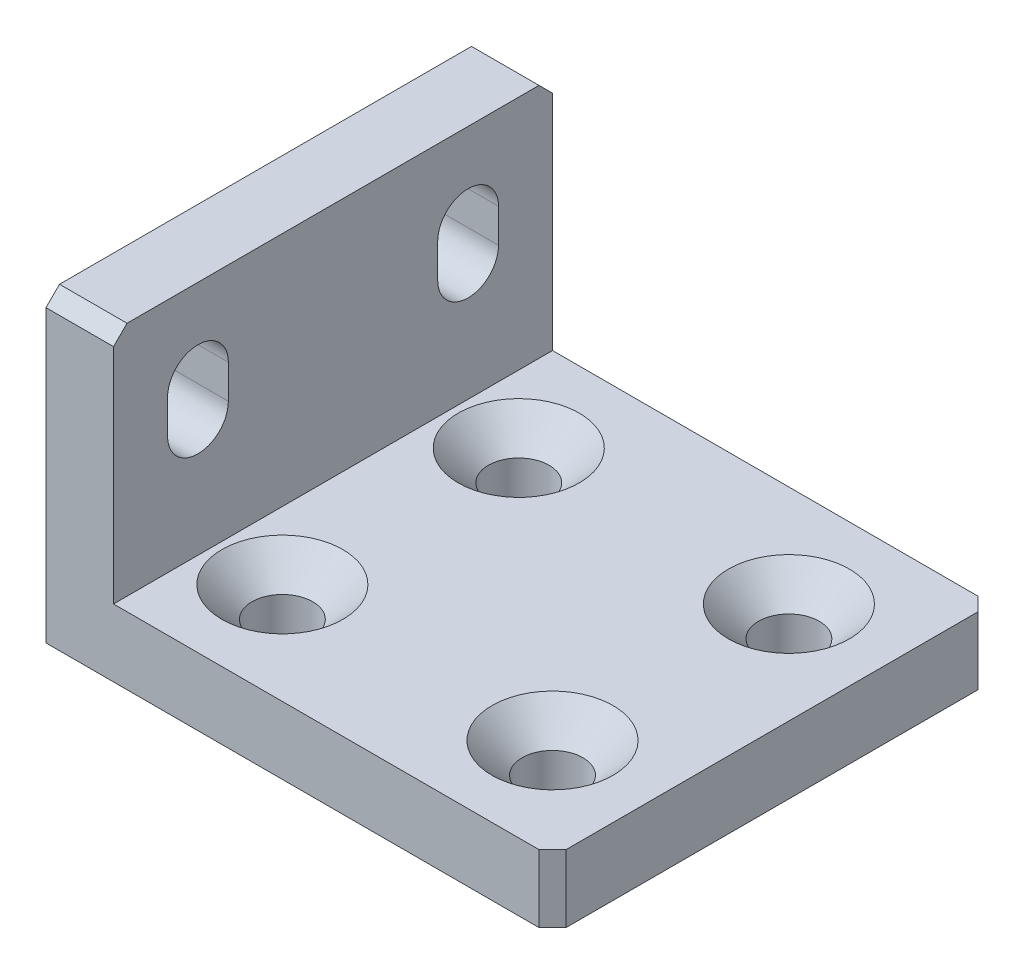
from build123d import *

# Parameters (mm, degrees)
SKETCH_2_W                   = 75
SKETCH_2_H                   = 65
EXTRUDE_1_DEPTH              = 5
SKETCH_3_W                   = 10
SKETCH_3_H                   = 65
EXTRUDE_2_DEPTH              = 45
HOLE_WIZARD_M8_1_D           = 9
HOLE_WIZARD_M8_1_CSINK_D     = 17.92
HOLE_WIZARD_M8_1_CSINK_ANGLE = 90
CUT_EXTRUDE_1_DEPTH          = 45
CHAMFER_1_SIZE               = 2


with BuildPart() as part:
    # 草图2 → 凸台-拉伸1 (new, symmetric)
    with BuildSketch(Plane(origin=(0, 0, 0), x_dir=(1, 0, 0), z_dir=(0, 1, 0))):
        Rectangle(SKETCH_2_W, SKETCH_2_H)
    extrude(amount=EXTRUDE_1_DEPTH, both=True)

    # 草图3 → 凸台-拉伸2 (add)
    with BuildSketch(Plane.XZ.offset(5)):
        with Locations((-32.5, 0)):
            Rectangle(SKETCH_3_W, SKETCH_3_H)
    extrude(amount=-EXTRUDE_2_DEPTH)

    # M8 六角凹锥坑螺钉的锥形沉头孔1 (through all)
    with Locations(Plane(origin=(0, 5, 0), x_dir=(1, 0, 0), z_dir=(0, 1, 0))):
        with Locations((22.5, 17.5), (-17.5, 17.5), (-17.5, -17.5), (22.5, -17.5)):
            CounterSinkHole(HOLE_WIZARD_M8_1_D / 2, HOLE_WIZARD_M8_1_CSINK_D / 2, counter_sink_angle=HOLE_WIZARD_M8_1_CSINK_ANGLE)

    # 草图6 → 切除-拉伸1 (cut)
    with BuildSketch(Plane(origin=(-27.5, 0, 0), x_dir=(0, 0, -1), z_dir=(1, 0, 0))):
        with BuildLine():
            Line((24.5, 27.5), (24.5, 22.5))
            ThreePointArc((24.5, 22.5), (20, 18), (15.5, 22.5))
            Line((15.5, 22.5), (15.5, 27.5))
            ThreePointArc((15.5, 27.5), (20, 32), (24.5, 27.5))
        make_face()
        with BuildLine():
            Line((-24.5, 27.5), (-24.5, 22.5))
            ThreePointArc((-24.5, 22.5), (-20, 18), (-15.5, 22.5))
            Line((-15.5, 22.5), (-15.5, 27.5))
            ThreePointArc((-15.5, 27.5), (-20, 32), (-24.5, 27.5))
        make_face()
    extrude(amount=-CUT_EXTRUDE_1_DEPTH, mode=Mode.SUBTRACT)

    # 倒角1
    chamfer_1_edges = [part.edges().sort_by_distance(p)[0] for p in [
        (-32.5, 40, -32.5),
        (-32.5, 40, 32.5),
        (37.5, 0, 32.5),
        (37.5, 0, -32.5),
    ]]
    chamfer(chamfer_1_edges, length=CHAMFER_1_SIZE)


solid = part.part
